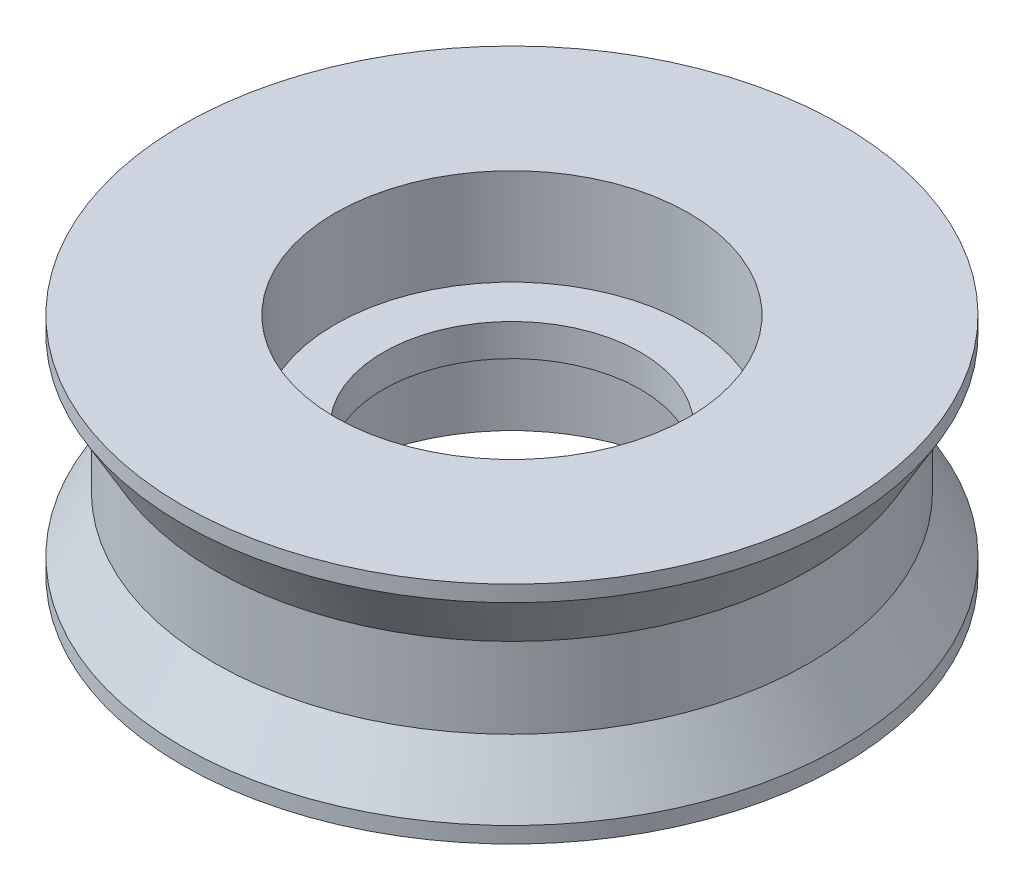
SolidWorks part; units mm, degrees
ref_plane "前视基准面" through (0, 0, 0) normal (0, 0, 1) x (1, 0, 0)
ref_plane "上视基准面" through (0, 0, 0) normal (0, 1, 0) x (1, 0, 0)
ref_plane "右视基准面" through (0, 0, 0) normal (1, 0, 0) x (0, 0, -1)
sketch "草图1" plane through (0, 0, 0) normal (0, 0, 1) x (1, 0, 0)
  line L0 (0, 20.6392) -> (0, -17.4107) construction
  line L1 (0, 0) -> (30.8312, 0) construction
  line L2 (20.5, -6) -> (18.5, -2.5)
  line L3 (11, -7) -> (20.5, -7)
  line L5 (11, 7) -> (20.5, 7)
  line L6 (20.5, -7) -> (20.5, -6)
  line L7 (18.5, -2.5) -> (18.5, 2.5)
  line L8 (20.5, 6) -> (18.5, 2.5)
  line L9 (20.5, 6) -> (20.5, 7)
  line L10 (11, -7) -> (11, -1)
  line L11 (11, -1) -> (8, -1)
  line L12 (8, -1) -> (8, 1)
  line L13 (8, 1) -> (11, 1)
  line L14 (11, 1) -> (11, 7)
  point P13 (18.5, 0)
  dimension "D1" = 14
  dimension "D2" = 20.5
  dimension "D3" = 1
  dimension "D4" = 18.5
  dimension "D5" = 2.5
  dimension "D6" = 6
  dimension "D7" = 11
  dimension "D8" = 3
revolve "旋转1" add sketch "草图1" angle 360 about L0
